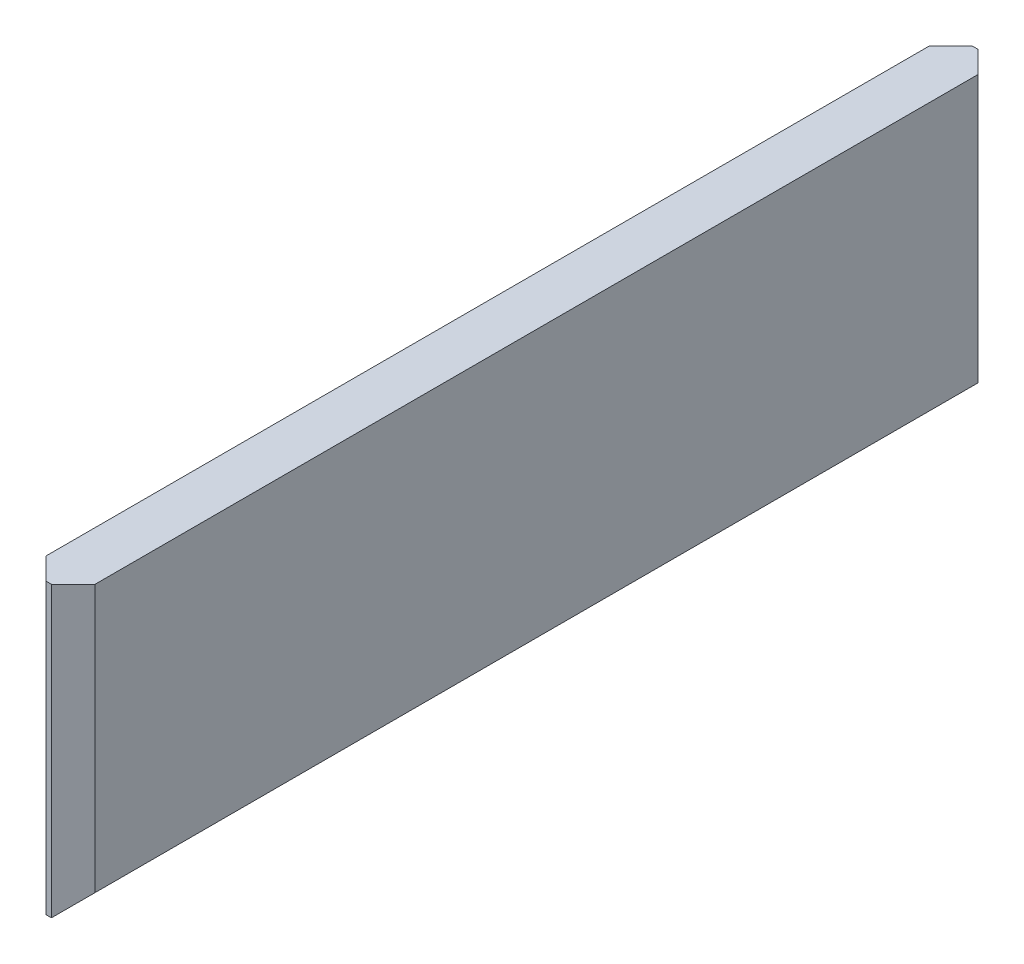
from build123d import *

# Parameters (mm, degrees)
SKETCH1_W           = 850
SKETCH1_H           = 265
BOSS_EXTRUDE1_DEPTH = 22.5
CHAMFER1_SIZE       = 20


with BuildPart() as part:
    # Sketch1 → Boss-Extrude1 (new, symmetric)
    with BuildSketch(Plane(origin=(0, 0, 0), x_dir=(0, 0, -1), z_dir=(1, 0, 0))):
        Rectangle(SKETCH1_W, SKETCH1_H)
    extrude(amount=BOSS_EXTRUDE1_DEPTH, both=True)

    # Chamfer1
    chamfer1_edges = [part.edges().sort_by_distance(p)[0] for p in [
        (22.5, 0, -425),
        (22.5, 0, 425),
        (-22.5, 0, -425),
        (-22.5, -132.5, 0),
        (-22.5, 0, 425),
        (22.5, -132.5, 0),
    ]]
    chamfer(chamfer1_edges, length=CHAMFER1_SIZE)


solid = part.part
